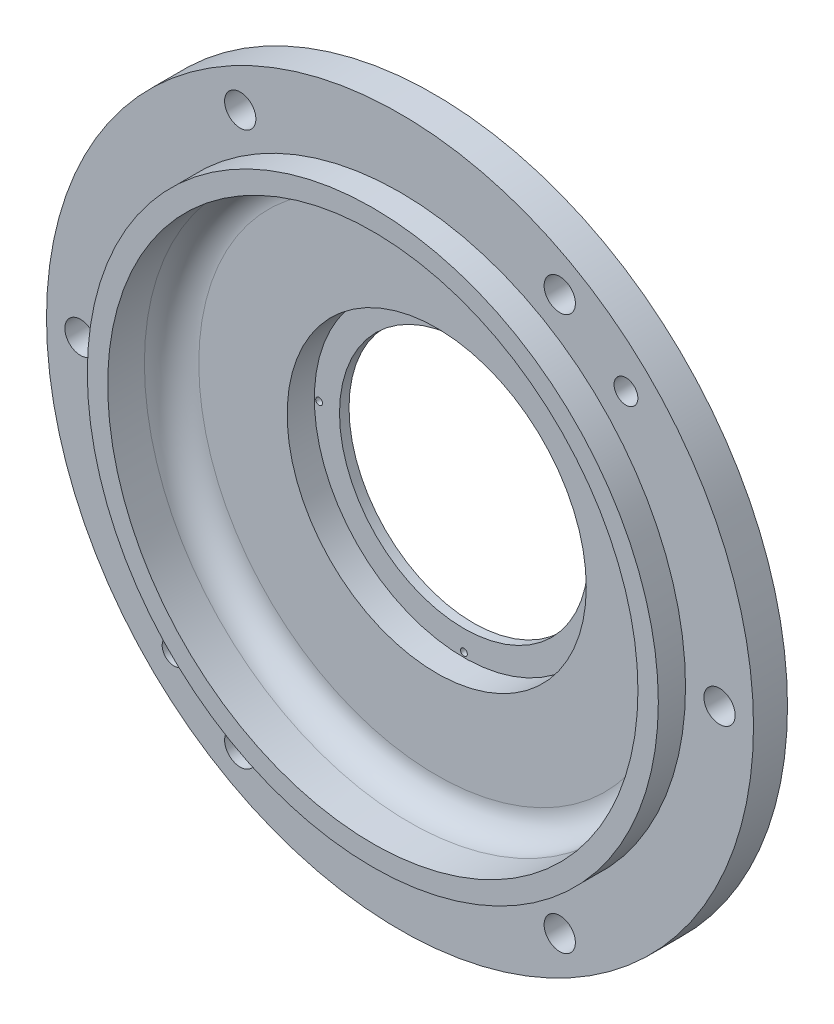
SolidWorks part; units mm, degrees
material "HT200"
ref_plane "Front Plane" through (0, 0, 0) normal (0, 0, 1) x (1, 0, 0)
ref_plane "Top Plane" through (0, 0, 0) normal (0, 1, 0) x (1, 0, 0)
ref_plane "Right Plane" through (0, 0, 0) normal (1, 0, 0) x (0, 0, -1)
sketch "Sketch1" plane through (0, 0, 0) normal (1, 0, 0) x (0, 0, -1)
  line L0 (0, 260) -> (25, 260)
  line L1 (25, 260) -> (25, 210)
  line L2 (25, 210) -> (29.7513, 210)
  line L3 (54, 168) -> (54, 91.5)
  line L4 (54, 91.5) -> (47, 91.5)
  line L5 (47, 91.5) -> (47, 110)
  line L6 (47, 110) -> (27, 110)
  line L7 (27, 110) -> (27, 195)
  line L8 (27, 195) -> (-20, 195)
  line L9 (-20, 195) -> (-20, 210)
  line L10 (-20, 210) -> (0, 210)
  line L11 (0, 210) -> (0, 260)
  line L12 (29.7513, 210) -> (54, 168)
  line L13 (-141.2331, 0) -> (214.5622, 0) construction
  dimension "D1" = 0
  dimension "D2" = 260
  dimension "D3" = 210
  dimension "D4" = 195
  dimension "D5" = 20
  dimension "D6" = 25
  dimension "D7" = 168
  dimension "D8" = 210
  dimension "D9" = 74
  dimension "D10" = 30
  dimension "D11" = 7
  dimension "D12" = 91.5
  dimension "D13" = 47
  dimension "D14" = 110
revolve "Revolve1" add sketch "Sketch1" angle 360 about L13
fillet "Fillet1" radius 20 1 edges at (195, 0, -27)
sketch "Sketch2" plane through (0, 0, -54) normal (0, 0, -1) x (-1, 0, 0)
  circle A0 centre (0, 106.5) radius 2.5
  dimension "D1" = 5
  dimension "D2" = 106.5
  dimension "D3" = 0
extrude "Cut-Extrude1" cut sketch "Sketch2" against normal up to next
pattern_circular "CirPattern1" count 4 over 360 about axis through (0, 0, 0) along (0, 0, 1) of "Cut-Extrude1"
sketch "Sketch3" plane through (0, 0, 0) normal (0, 0, 1) x (1, 0, 0)
  circle A0 centre (-235, 0) radius 11.5
  dimension "D1" = 23
  dimension "D2" = 235
  dimension "D3" = 0
extrude "Cut-Extrude2" cut sketch "Sketch3" against normal through all and the other way blind 5
pattern_circular "CirPattern2" count 6 over 360 about axis through (0, 0, 0) along (0, 0, 1) of "Cut-Extrude2"
hole_wizard "M20 Tapped Hole1" positions "Sketch5" profile "Sketch4" tap size "M20" standard "Gb" end condition through all
sketch "Sketch5" plane through (0, 0, 0) normal (0, 0, 1) x (1, 0, 0)
  line L0 (0, 0) -> (-166.1701, -166.1701) construction
  line L2 (0, 0) -> (-235, 0) construction
  circle A0 centre (0, 0) radius 235 construction
  point P0 (-166.1701, -166.1701)
  dimension "D2" = 470
  dimension "D1" = 45
sketch "Sketch4" plane through (-166.1701, -166.1701, 0) normal (1, 0, 0) x (0, -1, 0)
  line L0 (0, 0) -> (0, 54)
  line L1 (0, 54) -> (8.75, 54)
  line L2 (8.75, 54) -> (8.75, 0)
  line L5 (8.75, 0) -> (0, 0)
  line L11 (0, -6.35) -> (0, 107.95) construction
  dimension "通孔螺纹孔钻头直径" = 17.5
  dimension "通孔螺纹孔钻头深度" = 54
cosmetic thread "Cosmetic Thread1" parameters "D2"=20
pattern_circular "CirPattern3" count 2 over 360 about axis through (0, 0, 0) along (0, 0, 1) of "M20 Tapped Hole1"
hole_wizard "1/4 Rc Tapped Hole1" positions "3DSketch1" profile "Sketch6" size "1/4" standard "Gb" end condition through all
sketch3d "3DSketch1"
  line L0 (0, 0, 0) -> (0, 187.7452, -42.6001) construction
  line L2 (0, 0, 0) -> (-235, 0, 0) construction
  line L3 (-235, 0, 0) -> (-235, 0, -25) construction
  point P0 (0, 187.7452, -42.6001)
  dimension "D1" = 90
sketch "Sketch6" plane through (0, 187.7452, -42.6001) normal (1, 0, 0) x (0, 0.866, 0.5)
  line L0 (0, 0) -> (0, 278.0859)
  line L1 (0, 278.0859) -> (5.35, 278.0859)
  line L2 (-5.3791, 11) -> (-5.7225, 0) construction
  line L3 (5.35, 278.0859) -> (5.35, 11)
  line L4 (5.35, 11) -> (5.3791, 11)
  line L5 (5.3791, 11) -> (5.7225, 0)
  line L7 (5.7225, 0) -> (0, 0)
  line L8 (0, -6.35) -> (0, 107.95) construction
  line L11 (-5.35, 11) -> (-5.3791, 11) construction
  dimension "通孔螺纹孔钻头直径" = 10.7
  dimension "通孔螺纹孔钻头深度" = 278.0859
  dimension "螺纹直径" = 11.445
  dimension "螺纹角度" = 3.576
  dimension "螺纹深度" = 11
